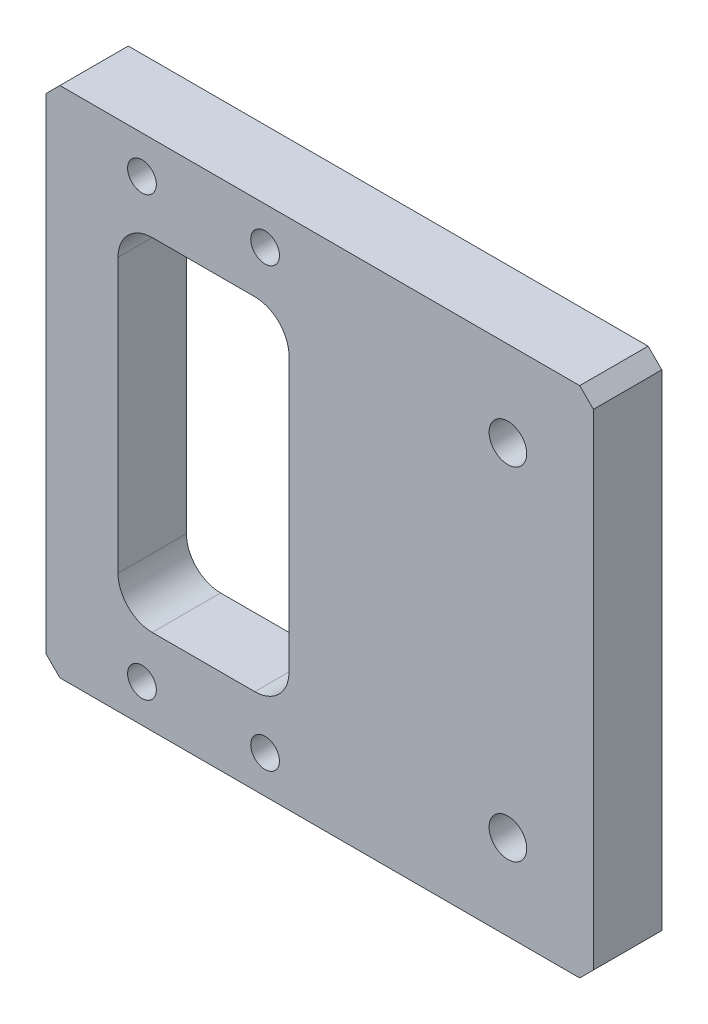
from build123d import *

# Parameters (mm, degrees)
SKETCH_1_W                   = 80
SKETCH_1_H                   = 75
EXTRUDE_1_DEPTH              = 5
CHAMFER_1_SIZE               = 2
HOLE_WIZARD_M5_1_D           = 5.5
HOLE_WIZARD_M5_1_CBORE_D     = 10
HOLE_WIZARD_M5_1_CBORE_DEPTH = 5.7
HOLE_WIZARD_M5_1_2_D         = 4.2
HOLE_WIZARD_M5_1_2_DEPTH     = 12.4
HOLE_WIZARD_M5_1_2_TIP       = 1.2618073
CUT_EXTRUDE_1_DEPTH          = 56.733742024


with BuildPart() as part:
    # 草图1 → 凸台-拉伸1 (new, symmetric)
    with BuildSketch(Plane.XY):
        Rectangle(SKETCH_1_W, SKETCH_1_H)
    extrude(amount=EXTRUDE_1_DEPTH, both=True)

    # 倒角1
    chamfer_1_edges = [part.edges().sort_by_distance(p)[0] for p in [
        (40, -37.5, 0),
        (-40, -37.5, 0),
        (-40, 37.5, 0),
        (40, 37.5, 0),
    ]]
    chamfer(chamfer_1_edges, length=CHAMFER_1_SIZE)

    # Hole Wizard M5 _1 (through all)
    with Locations(Plane(origin=(0, 0, -5), x_dir=(-1, 0, 0), z_dir=(0, 0, -1))):
        with Locations((-27.5, 25), (-27.5, -25)):
            CounterBoreHole(HOLE_WIZARD_M5_1_D / 2, HOLE_WIZARD_M5_1_CBORE_D / 2, HOLE_WIZARD_M5_1_CBORE_DEPTH)

    # Hole Wizard M5 _1 2
    with Locations(Plane(origin=(0, 0, -5), x_dir=(-1, 0, 0), z_dir=(0, 0, -1))):
        with Locations((7.999483419, 32), (25.999483419, 32), (7.999483419, -32), (25.999483419, -32)):
            Hole(HOLE_WIZARD_M5_1_2_D / 2, depth=HOLE_WIZARD_M5_1_2_DEPTH)
            with Locations((0, 0, -(HOLE_WIZARD_M5_1_2_DEPTH + HOLE_WIZARD_M5_1_2_TIP / 2))):  # 118° drill point
                Cone(0, HOLE_WIZARD_M5_1_2_D / 2, HOLE_WIZARD_M5_1_2_TIP, mode=Mode.SUBTRACT)

    # 草图8 → 切除-拉伸1 (cut, through all)
    with BuildSketch(Plane(origin=(0, 0, -5), x_dir=(-1, 0, 0), z_dir=(0, 0, -1))):
        with BuildLine():
            Line((9.499483419, -25), (24.499483419, -25))
            ThreePointArc((24.499483419, -25), (28.035017325, -23.535533906), (29.499483419, -20))
            Line((29.499483419, -20), (29.499483419, 20))
            ThreePointArc((29.499483419, 20), (28.035017325, 23.535533906), (24.499483419, 25))
            Line((24.499483419, 25), (9.499483419, 25))
            ThreePointArc((9.499483419, 25), (5.963949513, 23.535533906), (4.499483419, 20))
            Line((4.499483419, 20), (4.499483419, -20))
            ThreePointArc((4.499483419, -20), (5.963949513, -23.535533906), (9.499483419, -25))
        make_face()
    extrude(amount=-CUT_EXTRUDE_1_DEPTH, mode=Mode.SUBTRACT)


solid = part.part
